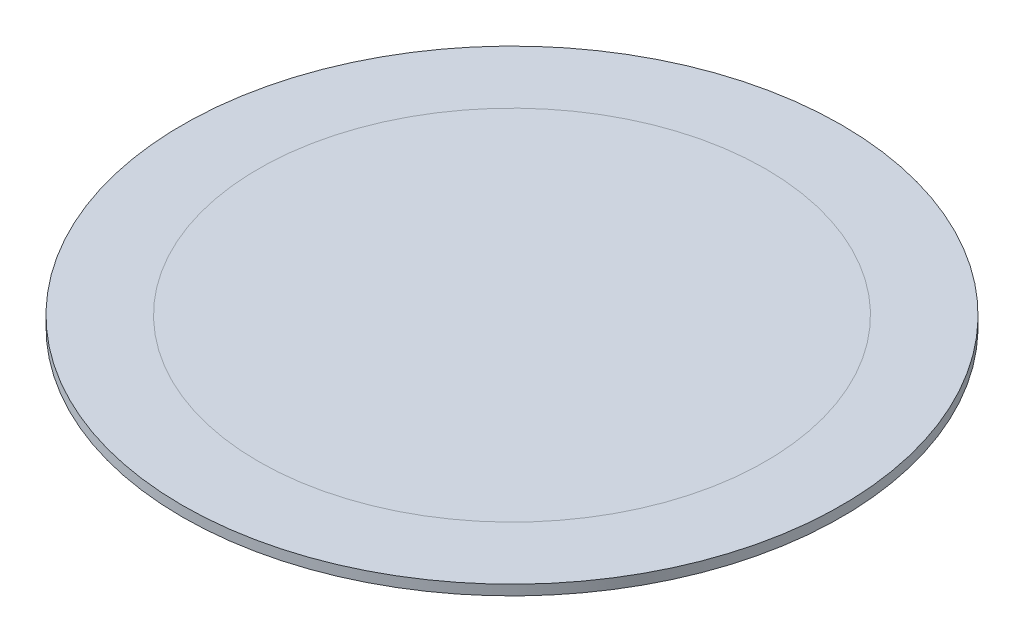
SolidWorks part; units mm, degrees
ref_plane "Front Plane" through (0, 0, 0) normal (0, 0, 1) x (1, 0, 0)
ref_plane "Top Plane" through (0, 0, 0) normal (0, 1, 0) x (1, 0, 0)
ref_plane "Right Plane" through (0, 0, 0) normal (1, 0, 0) x (0, 0, -1)
sketch "Sketch1" plane through (0, 0, 0) normal (0, 1, 0) x (1, 0, 0)
  circle A0 centre (0, 0) radius 25
  circle A1 centre (0, 0) radius 32.5
  dimension "D1" = 50
  dimension "D2" = 7.5
extrude "Boss-Extrude1" add sketch "Sketch1" along normal blind 1
sketch "Sketch2" plane through (0, 0, 0) normal (0, -1, 0) x (1, 0, 0)
  circle A0 centre (0, 0) radius 25 construction
  circle A1 centre (0, 0) radius 25
extrude "Boss-Extrude2" add sketch "Sketch2" against normal up to surface (1 mm away) separate body up to face at (0, 1, 32.5)
